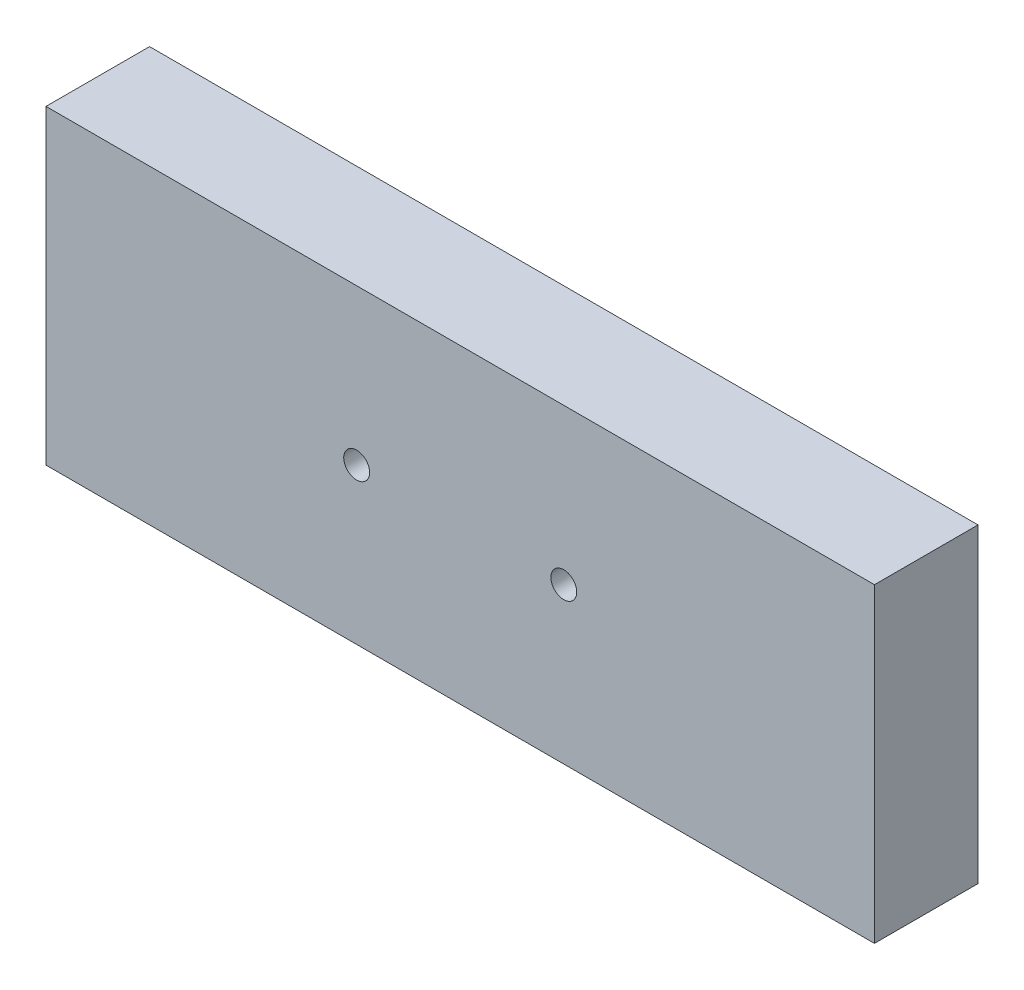
SolidWorks part; units mm, degrees
ref_plane "前视基准面" through (0, 0, 0) normal (0, 0, 1) x (1, 0, 0)
ref_plane "上视基准面" through (0, 0, 0) normal (0, 1, 0) x (1, 0, 0)
ref_plane "右视基准面" through (0, 0, 0) normal (1, 0, 0) x (0, 0, -1)
sketch "草图1" plane through (0, 0, 0) normal (0, 0, 1) x (1, 0, 0)
  line L1 (40, -15) -> (-40, -15)
  line L2 (40, -15) -> (40, 15)
  line L3 (40, 15) -> (-40, 15)
  line L4 (-40, -15) -> (-40, 15)
  line L5 (40, -15) -> (-40, 15) construction
  line L6 (40, 15) -> (-40, -15) construction
  point P0 (0, 0)
  point P5 (0, 0)
  dimension "D1" = 80
  dimension "D2" = 30
extrude "凸台-拉伸1" add sketch "草图1" along normal blind 10
sketch "草图2" plane through (0, 0, 10) normal (0, 0, 1) x (1, 0, 0)
  line L0 (-10, 0) -> (0, 0) construction
  line L1 (0, 0) -> (10, 0) construction
  circle A0 centre (-10, 0) radius 1.25
  circle A1 centre (10, 0) radius 1.25
  point P4 (0, 0)
  dimension "D2" = 2.5
  dimension "D1" = 10
extrude "切除-拉伸1" cut sketch "草图2" against normal blind 2
